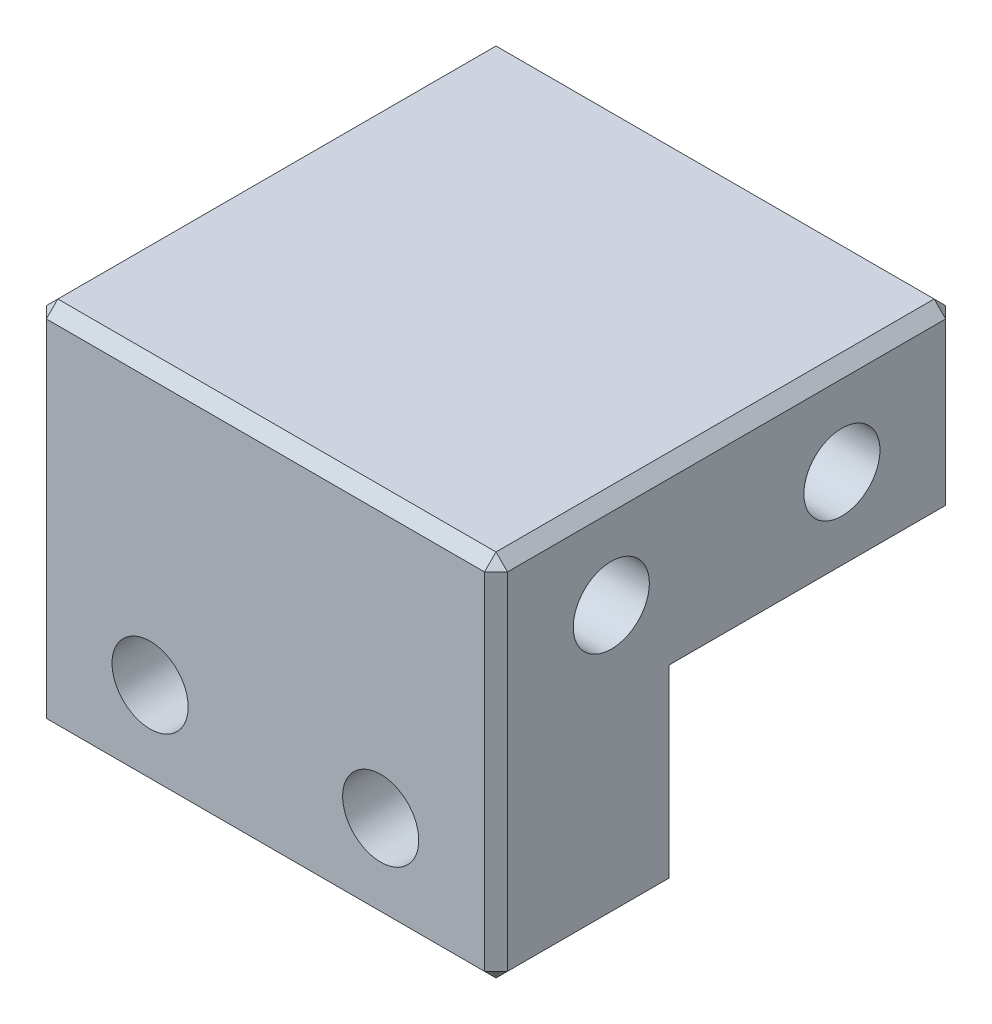
from build123d import *

# Parameters (mm, degrees)
SKETCH_1_W             = 20
SKETCH_1_H             = 20
EXTRUDE_1_DEPTH        = 8
HOLE_WIZARD_M4_1_D     = 3.3
HOLE_WIZARD_M4_1_DEPTH = 14.1
HOLE_WIZARD_M4_1_TIP   = 0.991420021
SKETCH_6_W             = 20
SKETCH_6_H             = 8
EXTRUDE_2_DEPTH        = 8
HOLE_WIZARD_M4_3_D     = 3.3
HOLE_WIZARD_M4_3_DEPTH = 14.1
HOLE_WIZARD_M4_3_TIP   = 0.991420021
CHAMFER_2_SIZE         = 0.5


with BuildPart() as part:
    # 草图1 → 凸台-拉伸1 (new body)
    with BuildSketch(Plane(origin=(0, 0, 0), x_dir=(1, 0, 0), z_dir=(0, 1, 0))):
        Rectangle(SKETCH_1_W, SKETCH_1_H)
    extrude(amount=EXTRUDE_1_DEPTH)

    # M4 螺纹孔1
    with Locations(Plane(origin=(10, 0, 0), x_dir=(0, 0, -1), z_dir=(1, 0, 0))):
        with Locations((5, 4), (-5, 4)):
            Hole(HOLE_WIZARD_M4_1_D / 2, depth=HOLE_WIZARD_M4_1_DEPTH)
            with Locations((0, 0, -(HOLE_WIZARD_M4_1_DEPTH + HOLE_WIZARD_M4_1_TIP / 2))):  # 118° drill point
                Cone(0, HOLE_WIZARD_M4_1_D / 2, HOLE_WIZARD_M4_1_TIP, mode=Mode.SUBTRACT)

    # 草图6 → 凸台-拉伸2 (add)
    with BuildSketch(Plane.XY.offset(10)):
        with Locations((0, -4)):
            Rectangle(SKETCH_6_W, SKETCH_6_H)
    extrude(amount=-EXTRUDE_2_DEPTH)

    # M4 螺纹孔3
    with Locations(Plane.XY.offset(10)):
        with Locations((-5, -4), (5, -4)):
            Hole(HOLE_WIZARD_M4_3_D / 2, depth=HOLE_WIZARD_M4_3_DEPTH)
            with Locations((0, 0, -(HOLE_WIZARD_M4_3_DEPTH + HOLE_WIZARD_M4_3_TIP / 2))):  # 118° drill point
                Cone(0, HOLE_WIZARD_M4_3_D / 2, HOLE_WIZARD_M4_3_TIP, mode=Mode.SUBTRACT)

    # 倒角2
    chamfer_2_edges = [part.edges().sort_by_distance(p)[0] for p in [
        (-10, 8, 0),
        (-10, 0, 10),
        (-10, -4, 2),
        (-10, 0, -4),
        (10, 4, -10),
        (0, 8, -10),
        (-10, 4, -10),
        (0, 0, -10),
        (10, -8, 6),
        (10, 0, -4),
        (10, -4, 2),
        (0, -8, 2),
        (-10, -8, 6),
        (0, -8, 10),
        (10, 8, 0),
        (0, 8, 10),
        (10, 0, 10),
    ]]
    chamfer(chamfer_2_edges, length=CHAMFER_2_SIZE)


solid = part.part
